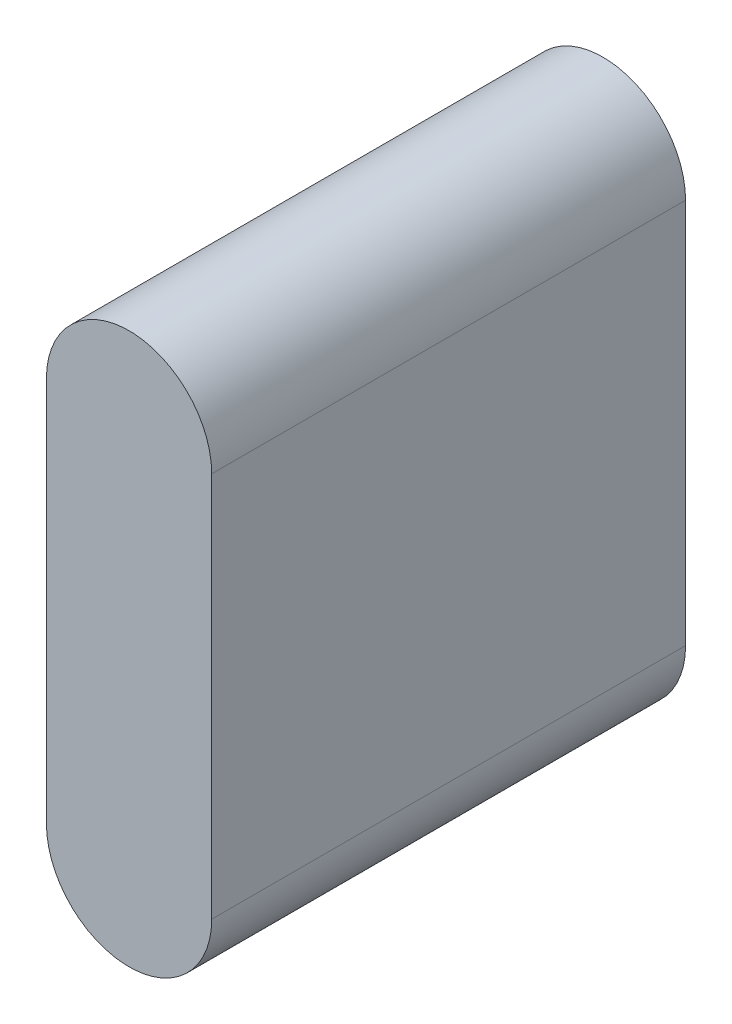
SolidWorks part; units mm, degrees
ref_plane "前视基准面" through (0, 0, 0) normal (0, 0, 1) x (1, 0, 0)
ref_plane "上视基准面" through (0, 0, 0) normal (0, 1, 0) x (1, 0, 0)
ref_plane "右视基准面" through (0, 0, 0) normal (1, 0, 0) x (0, 0, -1)
sketch "草图1" plane through (0, 0, 0) normal (0, 0, 1) x (1, 0, 0)
  line L0 (0, -1.75) -> (0, 1.75) construction
  line L1 (-0.75, -1.75) -> (-0.75, 1.75)
  line L2 (0.75, -1.75) -> (0.75, 1.75)
  arc A0 (-0.75, -1.75) -> (0.75, -1.75) centre (0, -1.75) ccw
  arc A1 (0.75, 1.75) -> (-0.75, 1.75) centre (0, 1.75) ccw
  point P3 (0, 0)
  dimension "D2" = 5
  dimension "D1" = 1.5
extrude "凸台-拉伸1" add sketch "草图1" along normal mid plane 4.3
